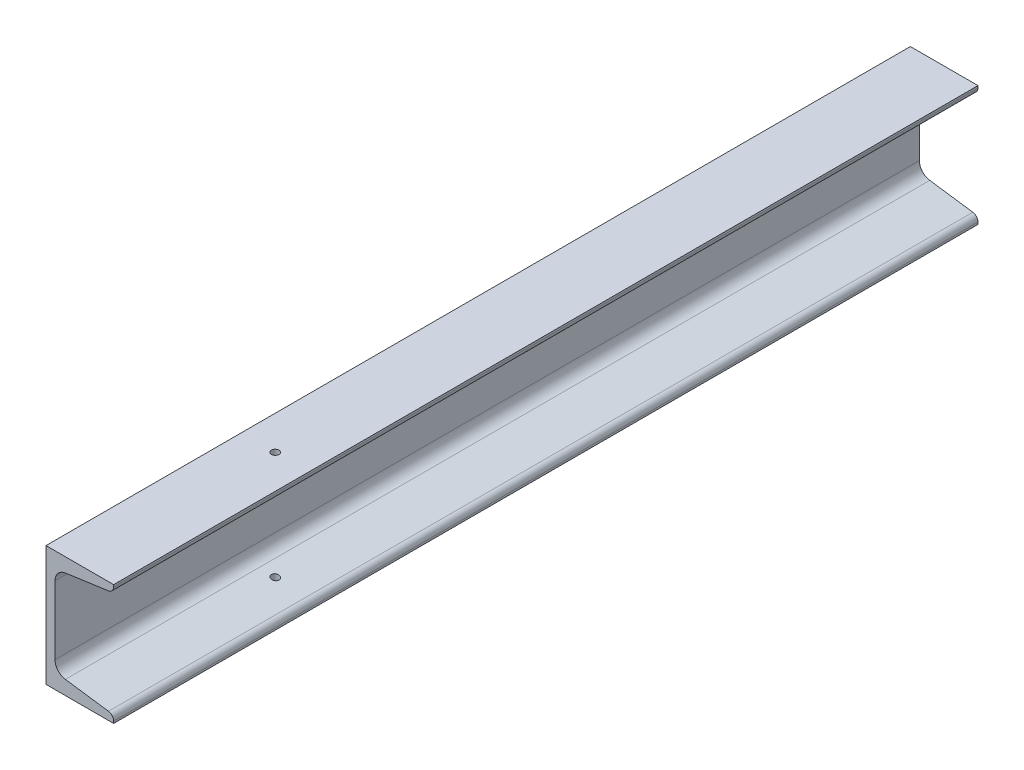
from build123d import *

# Parameters (mm, degrees)
EXTRUDE_1_DEPTH    = 575
HOLE_WIZARD_M6_1_D = 5


with BuildPart() as part:
    # 草图1 → 凸台-拉伸1 (new body)
    with BuildSketch(Plane.XY):
        with BuildLine():
            Line((0, 0), (-45, 0))
            Line((-45, 0), (-45, -80))
            Line((-45, -80), (0, -80))
            Line((0, -80), (0, -78.639315732))
            ThreePointArc((0, -78.639315732), (-0.981161679, -76.015079616), (-3.443307596, -74.678243457))
            Line((-3.443307596, -74.678243457), (-32.113384808, -70.648926875))
            ThreePointArc((-32.113384808, -70.648926875), (-37.037676642, -67.975254557), (-39, -62.726782325))
            Line((-39, -62.726782325), (-39, -17.273217675))
            ThreePointArc((-39, -17.273217675), (-37.037676642, -12.024745443), (-32.113384808, -9.351073125))
            Line((-32.113384808, -9.351073125), (-3.443307596, -5.321756543))
            ThreePointArc((-3.443307596, -5.321756543), (-0.981161679, -3.984920384), (0, -1.360684268))
            Line((0, -1.360684268), (0, 0))
        make_face()
    extrude(amount=EXTRUDE_1_DEPTH)

    # M6 螺纹孔1 (through all)
    with Locations(Plane(origin=(0, -80, 0), x_dir=(-1, 0, 0), z_dir=(0, -1, 0))):
        with Locations((22.5, -445)):
            Hole(HOLE_WIZARD_M6_1_D / 2)


solid = part.part
